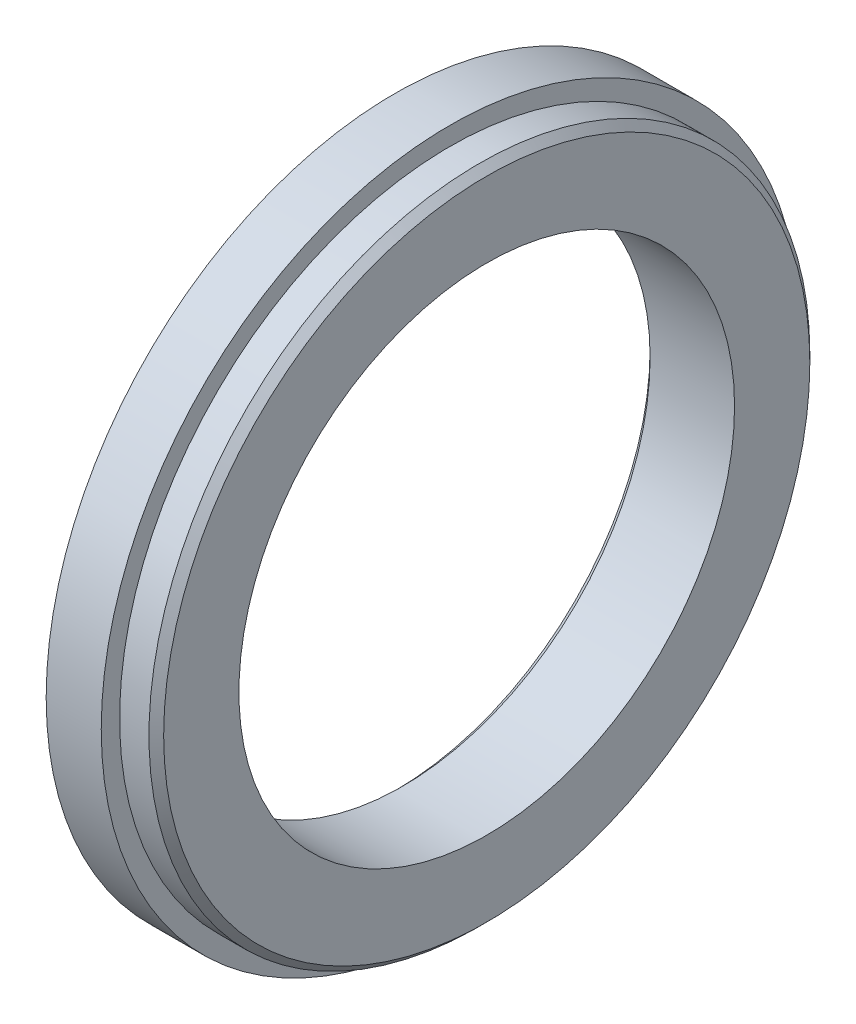
from build123d import *

# Parameters (mm, degrees)
SKETCH1_R           = 95
SKETCH1_R_2         = 67.5
BOSS_EXTRUDE1_DEPTH = 25
CUT_EXTRUDE1_START  = -10
SKETCH2_R           = 95
SKETCH2_R_2         = 90
CUT_EXTRUDE1_DEPTH  = 10
SKETCH3_R           = 5.75
CUT_EXTRUDE2_DEPTH  = 17.5
CHAMFER1_SIZE       = 2


with BuildPart() as part:
    # Sketch1 → Boss-Extrude1 (new body)
    with BuildSketch(Plane(origin=(0, 0, 0), x_dir=(0, 0, -1), z_dir=(1, 0, 0))):
        Circle(SKETCH1_R)
        Circle(SKETCH1_R_2, mode=Mode.SUBTRACT)
    extrude(amount=BOSS_EXTRUDE1_DEPTH)

    # Sketch2 → Cut-Extrude1 (cut)
    with BuildSketch(Plane(origin=(25, 0, 0), x_dir=(0, 0, -1), z_dir=(1, 0, 0)).offset(CUT_EXTRUDE1_START)):
        Circle(SKETCH2_R)
        Circle(SKETCH2_R_2, mode=Mode.SUBTRACT)
    extrude(amount=CUT_EXTRUDE1_DEPTH, mode=Mode.SUBTRACT)

    # Sketch3 → Cut-Extrude2 (cut)
    with BuildSketch(Plane.ZY):
        with Locations((40.25, -69.715045005)):
            Circle(SKETCH3_R)
        with Locations((80.5, 0)):
            Circle(SKETCH3_R)
        with Locations((-40.25, -69.715045005)):
            Circle(SKETCH3_R)
        with Locations((-80.5, 0)):
            Circle(SKETCH3_R)
        with Locations((-40.25, 69.715045005)):
            Circle(SKETCH3_R)
        with Locations((40.25, 69.715045005)):
            Circle(SKETCH3_R)
    extrude(amount=-CUT_EXTRUDE2_DEPTH, mode=Mode.SUBTRACT)

    # Chamfer1
    chamfer1_edges = [part.edges().sort_by_distance(p)[0] for p in [
        (25, 0, 90),
        (0, 0, 67.5),
    ]]
    chamfer(chamfer1_edges, length=CHAMFER1_SIZE)


solid = part.part
